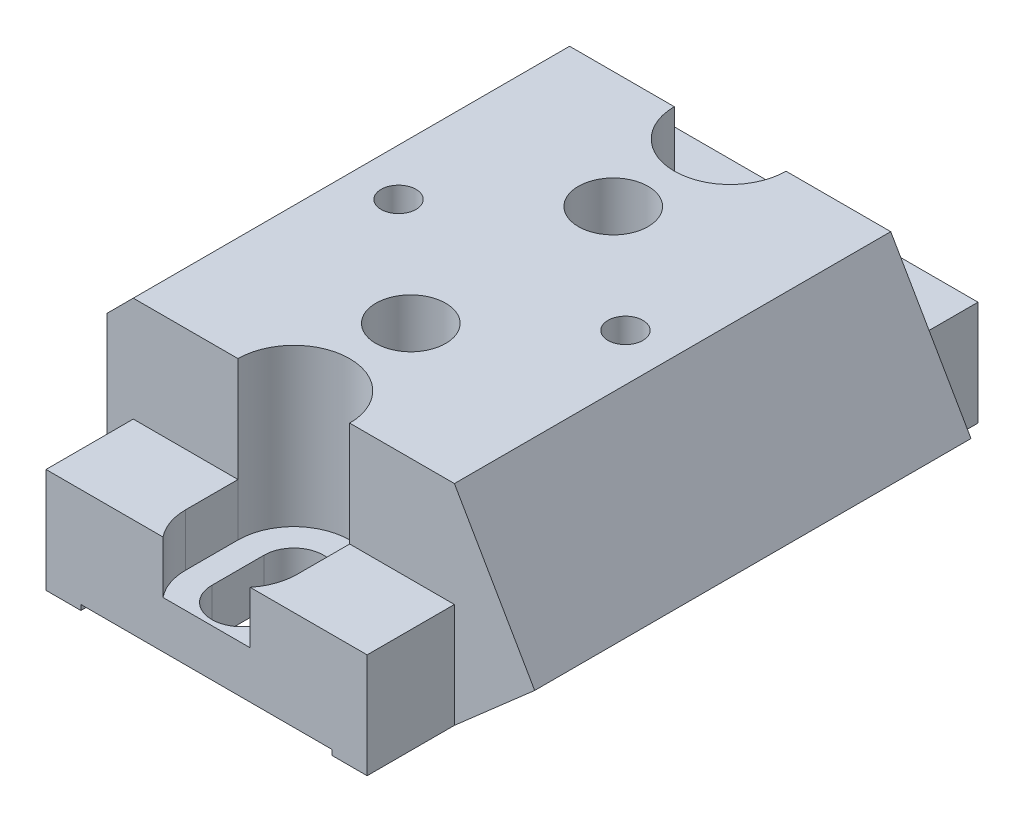
SolidWorks part; units mm, degrees
ref_plane "Front Plane" through (0, 0, 0) normal (0, 0, 1) x (1, 0, 0)
ref_plane "Top Plane" through (0, 0, 0) normal (0, 1, 0) x (1, 0, 0)
ref_plane "Right Plane" through (0, 0, 0) normal (1, 0, 0) x (0, 0, -1)
sketch "Sketch1" plane through (0, 0, 0) normal (0, 0, 1) x (1, 0, 0)
  line L1 (0, 0) -> (25, 0)
  line L2 (0, 0) -> (0, -12)
  line L3 (0, -12) -> (25, -12)
  line L4 (25, 0) -> (25, -12)
extrude "Boss-Extrude1" add sketch "Sketch1" along normal blind 25
sketch "Sketch2" plane through (0, 0, 25) normal (0, 0, 1) x (1, 0, 0)
  line L2 (25, 0) -> (25, -7.9674)
  line L3 (25, -12) -> (25, 0) construction
  line L5 (25, -7.9674) -> (20.4, 0)
  line L7 (25, 0) -> (20.4, 0)
  line L8 (25, 0) -> (0, 0) construction
  dimension "D1" = 30
extrude "Cut-Extrude1" cut sketch "Sketch2" against normal blind 30
chamfer "Chamfer1" distance 2 angle 45 3 edges at (0, -12, 12.5) (25, -12, 12.5) (0, 0, 12.5)
sketch "Sketch5" plane through (0, -12, 0) normal (0, -1, 0) x (1, 0, 0)
  line L10 (2, 30) -> (23, 30)
  line L11 (2, 30) -> (2, -5)
  line L12 (2, -5) -> (23, -5)
  line L13 (23, 30) -> (23, -5)
extrude "Boss-Extrude2" add sketch "Sketch5" against normal blind 6
sketch "Sketch6" plane through (0, -6, 0) normal (0, 1, 0) x (1, 0, 0)
  line L1 (20.4, -25) -> (23, -25)
  line L2 (20.4, -25) -> (20.4, -30)
  line L3 (20.4, -30) -> (23, -30)
  line L4 (23, -25) -> (23, -30)
  line L5 (23, 5) -> (20.4, 5)
  line L6 (23, 5) -> (23, 0)
  line L7 (23, 0) -> (20.4, 0)
  line L8 (20.4, 5) -> (20.4, 0)
extrude "Cut-Extrude2" cut sketch "Sketch6" against normal blind 10
sketch "Sketch11" plane through (0, 0, 30) normal (0, 0, 1) x (1, 0, 0)
  line L0 (20.4, -12) -> (2, -12) construction
  line L1 (4, -12) -> (18.4, -12)
  line L2 (4, -12) -> (4, -11.7)
  line L3 (4, -11.7) -> (18.4, -11.7)
  line L4 (18.4, -12) -> (18.4, -11.7)
  line L5 (2, -6) -> (2, -12) construction
  line L6 (20.4, -12) -> (20.4, -6) construction
  dimension "D1" = 2
  dimension "D2" = 2
  dimension "D3" = 0.3
extrude "Cut-Extrude5" cut sketch "Sketch11" against normal blind 48
sketch "Sketch12" plane through (0, 0, 30) normal (0, 0, 1) x (1, 0, 0)
  line L0 (25, -7.9674) -> (20.4, -12)
  line L1 (20.4, -12) -> (25.5929, -12)
  line L2 (25.5929, -12) -> (25, -7.9674)
extrude "Cut-Extrude6" cut sketch "Sketch12" against normal blind 48
sketch "Sketch15" plane through (0, 0, 0) normal (-1, 0, 0) x (0, 0, 1)
  line L1 (0, 0) -> (25, 0)
  line L2 (0, 0) -> (0, -12)
  line L3 (0, -12) -> (25, -12)
  line L4 (25, 0) -> (25, -12)
extrude "Cut-Extrude8" cut sketch "Sketch15" against normal blind 0.5
sketch "Sketch17" plane through (0, 0, 0) normal (0, 1, 0) x (1, 0, 0)
  line L0 (20.4, 0) -> (2, 0) construction
  line L1 (20.4, -25) -> (2, -25) construction
  line L2 (2, 0) -> (2, -25) construction
  circle A0 centre (11.2, -6.7) radius 2
  circle A1 centre (11.2, -18.3) radius 2
  dimension "D1" = 6.7
  dimension "D2" = 6.7
  dimension "D3" = 9.2
  dimension "D4" = 4
  dimension "D5" = 9.2
extrude "Cut-Extrude10" cut sketch "Sketch17" against normal blind 5
sketch "Sketch18" plane through (0, 0, 0) normal (0, 1, 0) x (1, 0, 0)
  line L0 (2, -12.5) -> (20.4, -12.5) construction
  line L1 (2, 0) -> (2, -25) construction
  line L2 (20.4, 0) -> (20.4, -25) construction
  circle A0 centre (4.7, -12.5) radius 1
  circle A1 centre (17.7, -12.5) radius 1
  circle A2 centre (11.2, -6.7) radius 2 construction
  dimension "D1" = 6.5
  dimension "D2" = 13
extrude "Cut-Extrude11" cut sketch "Sketch18" against normal blind 4
sketch "Sketch19" plane through (0, 0, 0) normal (0, 1, 0) x (1, 0, 0)
  line L0 (11.2, -25) -> (11.2, -28) construction
  line L1 (20.4, -25) -> (2, -25) construction
  line L2 (12.9, -25) -> (12.9, -28)
  line L3 (9.5, -25) -> (9.5, -28)
  line L4 (-998, -12.5) -> (49002, -12.5) construction
  line L5 (2, 0) -> (2, -25) construction
  line L7 (11.2, 0) -> (11.2, 3) construction
  line L8 (12.9, 0) -> (12.9, 3)
  line L9 (9.5, 0) -> (9.5, 3)
  arc A0 (12.9, -25) -> (9.5, -25) centre (11.2, -25) ccw
  arc A1 (9.5, -28) -> (12.9, -28) centre (11.2, -28) ccw
  arc A2 (12.9, 0) -> (9.5, 0) centre (11.2, 0) cw
  arc A3 (9.5, 3) -> (12.9, 3) centre (11.2, 3) cw
  point P4 (11.2, -26.5)
  point P14 (2, -12.5)
  point P16 (11.2, 1.5)
  dimension "D1" = 1.7
  dimension "D2" = 3
extrude "Cut-Extrude12" cut sketch "Sketch19" against normal blind 17
sketch "Sketch20" plane through (0, 0, 0) normal (0, 1, 0) x (1, 0, 0)
  line L0 (11.2, -25) -> (11.2, -28) construction
  line L1 (14.4, -25) -> (14.4, -28)
  line L2 (8, -25) -> (8, -28)
  line L4 (-998, -12.5) -> (49002, -12.5) construction
  line L5 (2, 0) -> (2, -25) construction
  line L6 (11.2, 0) -> (11.2, 3) construction
  line L7 (14.4, 0) -> (14.4, 3)
  line L8 (8, 0) -> (8, 3)
  arc A0 (14.4, -25) -> (8, -25) centre (11.2, -25) ccw
  arc A1 (8, -28) -> (14.4, -28) centre (11.2, -28) ccw
  arc A2 (14.4, 0) -> (8, 0) centre (11.2, 0) cw
  arc A3 (8, 3) -> (14.4, 3) centre (11.2, 3) cw
  point P3 (11.2, -26.5)
  point P13 (2, -12.5)
  point P15 (11.2, 1.5)
  dimension "D1" = 3.2
  dimension "D2" = 3
extrude "Cut-Extrude13" cut sketch "Sketch20" against normal blind 9
